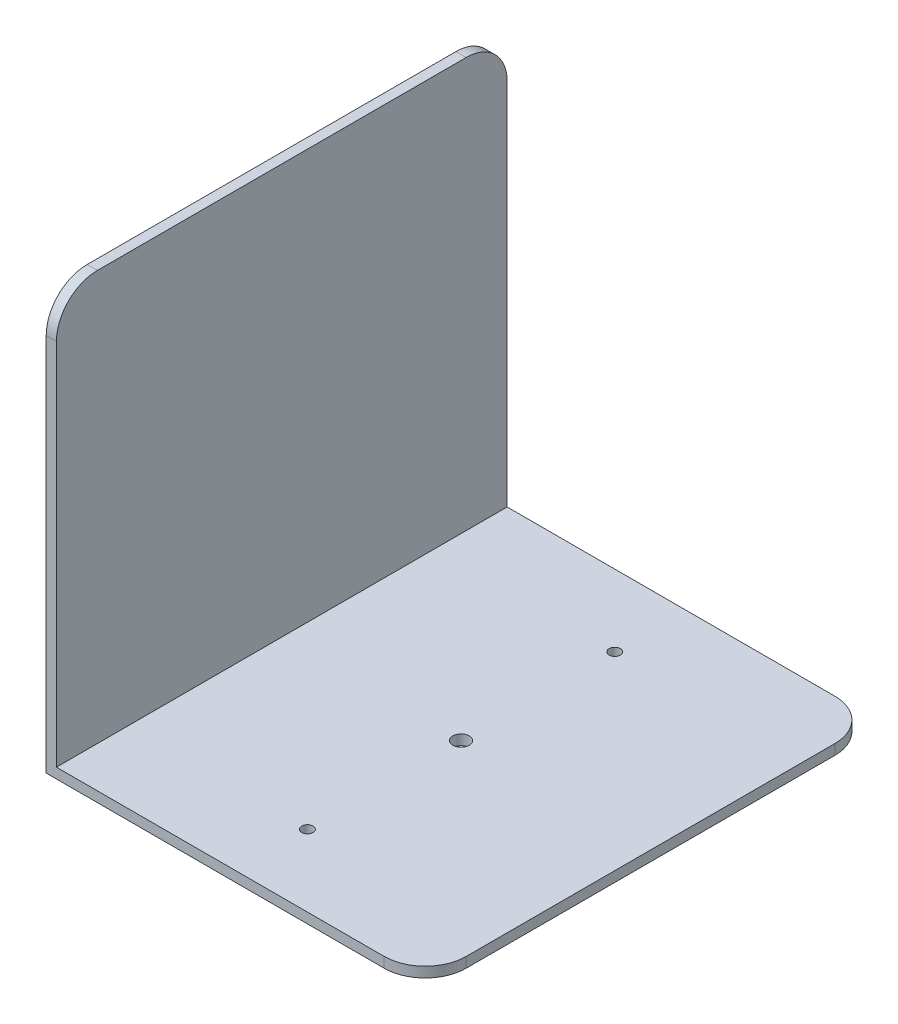
SolidWorks part; units mm, degrees
material "PVC 0.007 塑化"
ref_plane "前视基准面" through (0, 0, 0) normal (0, 0, 1) x (1, 0, 0)
ref_plane "上视基准面" through (0, 0, 0) normal (0, 1, 0) x (1, 0, 0)
ref_plane "右视基准面" through (0, 0, 0) normal (1, 0, 0) x (0, 0, -1)
sketch "草图1" plane through (0, 0, 0) normal (0, 1, 0) x (1, 0, 0)
  line L1 (-185, 220) -> (185, 220)
  line L2 (-185, 220) -> (-185, -220)
  line L3 (-185, -220) -> (185, -220)
  line L4 (185, 220) -> (185, -220)
  line L5 (-185, 220) -> (185, -220) construction
  line L6 (-185, -220) -> (185, 220) construction
  point P0 (0, 0)
  dimension "D1" = 440
  dimension "D2" = 370
extrude "凸台-拉伸1" add sketch "草图1" along normal mid plane 10
sketch "草图2" plane through (0, 5, 0) normal (0, 1, 0) x (1, 0, 0)
  line L0 (-5.5, 0) -> (5.5, 0) construction
  circle A0 centre (0, 0) radius 8
  circle A1 centre (0, 150) radius 5.5
  circle A2 centre (0, -150) radius 5.5
  dimension "D1" = 16
  dimension "D2" = 300
  dimension "D3" = 11
extrude "切除-拉伸1" cut sketch "草图2" against normal up to next
sketch "草图3" plane through (0, 5, 0) normal (0, 1, 0) x (1, 0, 0)
  line L0 (-185, -220) -> (185, -220) construction
  line L1 (-185, 220) -> (-175, 220)
  line L2 (-185, 220) -> (-185, -220)
  line L3 (-185, -220) -> (-175, -220)
  line L4 (-175, 220) -> (-175, -220)
  dimension "D1" = 10
extrude "凸台-拉伸2" add sketch "草图3" along normal blind 400
fillet "圆角1" radius 40 4 edges at (185, 0, -220) (185, 0, 220) (-180, 405, -220) (-180, 405, 220)
